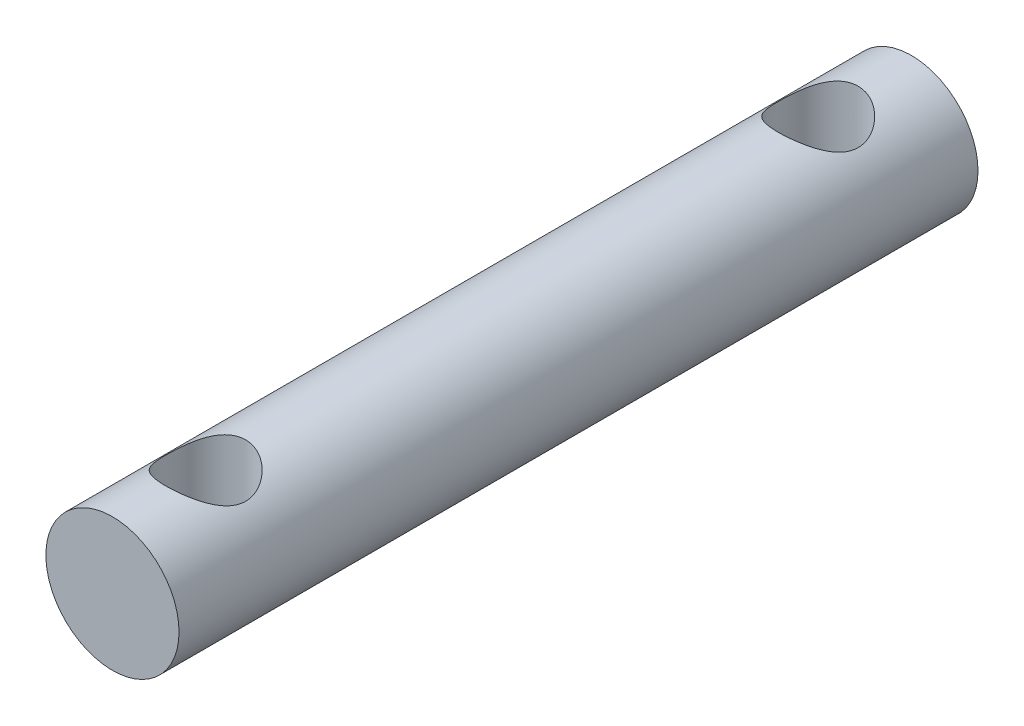
from build123d import *

# Parameters (mm, degrees)
SKETCH1_R               = 5
BOSS_EXTRUDE1_DEPTH     = 60
CUT_EXTRUDE1_DEPTH      = 61.415229868
CUT_EXTRUDE1_DEPTH_BACK = 61.415229868
SKETCH2_R               = 3


with BuildPart() as part:
    # Sketch1 → Boss-Extrude1 (new body)
    with BuildSketch(Plane.XY):
        Circle(SKETCH1_R)
    extrude(amount=BOSS_EXTRUDE1_DEPTH)

    # Sketch2 → Cut-Extrude1 (cut, two sides: drawn at the far end of the back side and taken through both)
    with BuildSketch(Plane(origin=(0, 0, 0), x_dir=(1, 0, 0), z_dir=(0, 1, 0)).offset(-CUT_EXTRUDE1_DEPTH_BACK)):
        with Locations(Location((0, -7, 0), (0, 0, 270))):
            Circle(SKETCH2_R)
        with Locations(Location((0, -53, 0), (0, 0, 270))):
            Circle(SKETCH2_R)
    extrude(amount=CUT_EXTRUDE1_DEPTH + CUT_EXTRUDE1_DEPTH_BACK, mode=Mode.SUBTRACT)


solid = part.part
